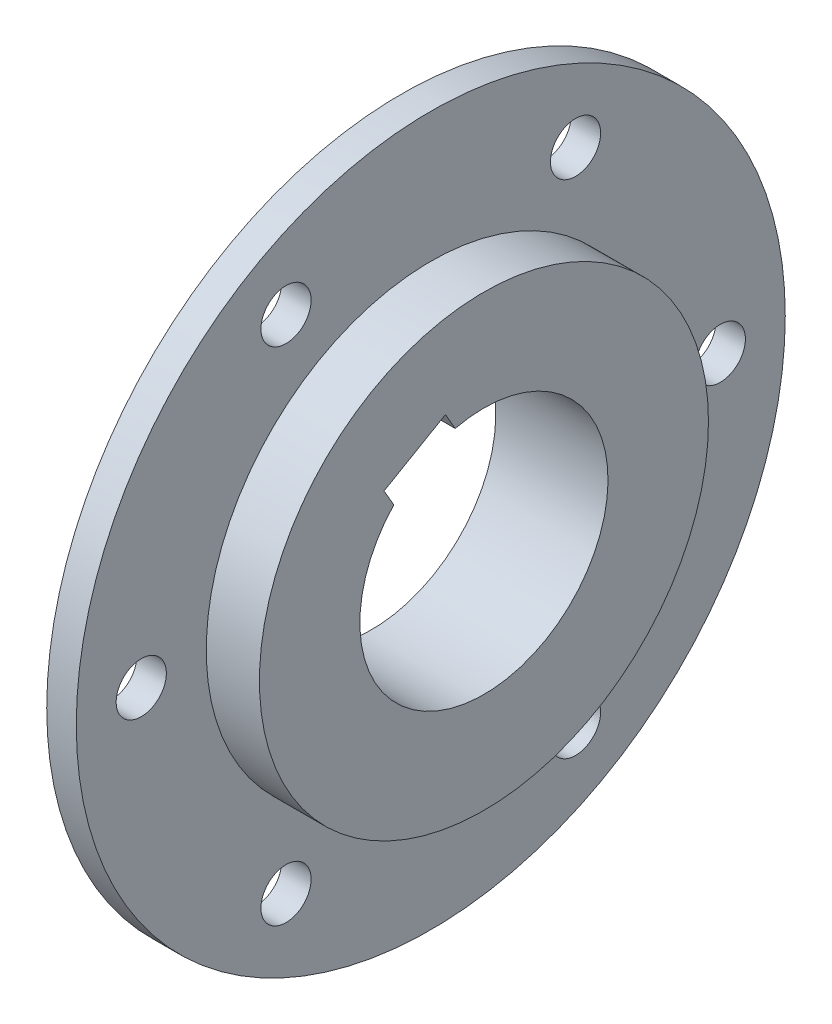
SolidWorks part; units mm, degrees
ref_plane "前视基准面" through (0, 0, 0) normal (0, 0, 1) x (1, 0, 0)
ref_plane "上视基准面" through (0, 0, 0) normal (0, 1, 0) x (1, 0, 0)
ref_plane "右视基准面" through (0, 0, 0) normal (1, 0, 0) x (0, 0, -1)
sketch "草图1" plane through (0, 0, 0) normal (1, 0, 0) x (0, 0, -1)
  line L0 (0, 0) -> (0, 50.7496) construction
  line L2 (-4.8662, 20.4284) -> (-6.5162, 23.2863)
  line L3 (-6.5162, 23.2863) -> (-16.9085, 17.2863)
  line L4 (-16.9085, 17.2863) -> (-15.2585, 14.4284)
  arc A0 (-15.2585, 14.4284) -> (-4.8662, 20.4284) centre (0, 0) ccw
  circle A1 centre (0, 0) radius 38
  dimension "D1" = 3.3
extrude "凸台-拉伸1" add sketch "草图1" along normal blind 14 and the other way blind 5
sketch "草图2" plane through (0, 0, 0) normal (1, 0, 0) x (0, 0, -1)
  circle A0 centre (0, 0) radius 38
  circle A2 centre (0, 0) radius 60
extrude "凸台-拉伸2" add sketch "草图2" along normal blind 5
chamfer "倒角1" distance 1 angle 45 1 edges at (-5, 0, -38)
hole_wizard "M10 螺纹孔1" positions "草图7" profile "草图6" tap size "M10" standard "Iso"
sketch "草图7" plane through (0, 0, 0) normal (-1, 0, 0) x (0, 0, 1)
  line L0 (0, 0) -> (25000, 43301.2702) construction
  line L1 (0, 0) -> (25000, -43301.2702) construction
  line L2 (0, 0) -> (50000, 0) construction
  circle A0 centre (0, 0) radius 49 construction
  point P0 (24.5, 42.4352)
  point P23 (49, 0)
  point P25 (24.5, -42.4352)
  point P27 (-24.5, -42.4352)
  point P29 (-49, 0)
  point P31 (-24.5, 42.4352)
  dimension "D1" = 60
  dimension "D2" = 60
sketch "草图6" plane through (0, 42.4352, 24.5) normal (0, 1, 0) x (0, 0, 1)
  line L0 (0, 0) -> (0, 27.0537)
  line L1 (0, 27.0537) -> (4.25, 24.5)
  line L2 (4.25, 24.5) -> (4.25, 0)
  line L5 (4.25, 0) -> (0, 0)
  line L10 (0, 27.0537) -> (-4.25, 24.5) construction
  line L11 (0, -6.35) -> (0, 107.95) construction
  dimension "螺纹孔钻头直径" = 8.5
  dimension "螺纹孔钻头深度" = 24.5
  dimension "导头角度" = 118
cosmetic thread "孔螺蚊线7" parameters "D1"=5, "D2"=10
cosmetic thread "孔螺蚊线8" parameters "D1"=5, "D2"=10
cosmetic thread "孔螺蚊线9" parameters "D1"=5, "D2"=10
cosmetic thread "孔螺蚊线10" parameters "D1"=5, "D2"=10
cosmetic thread "孔螺蚊线11" parameters "D1"=5, "D2"=10
cosmetic thread "孔螺蚊线12" parameters "D1"=5, "D2"=10
